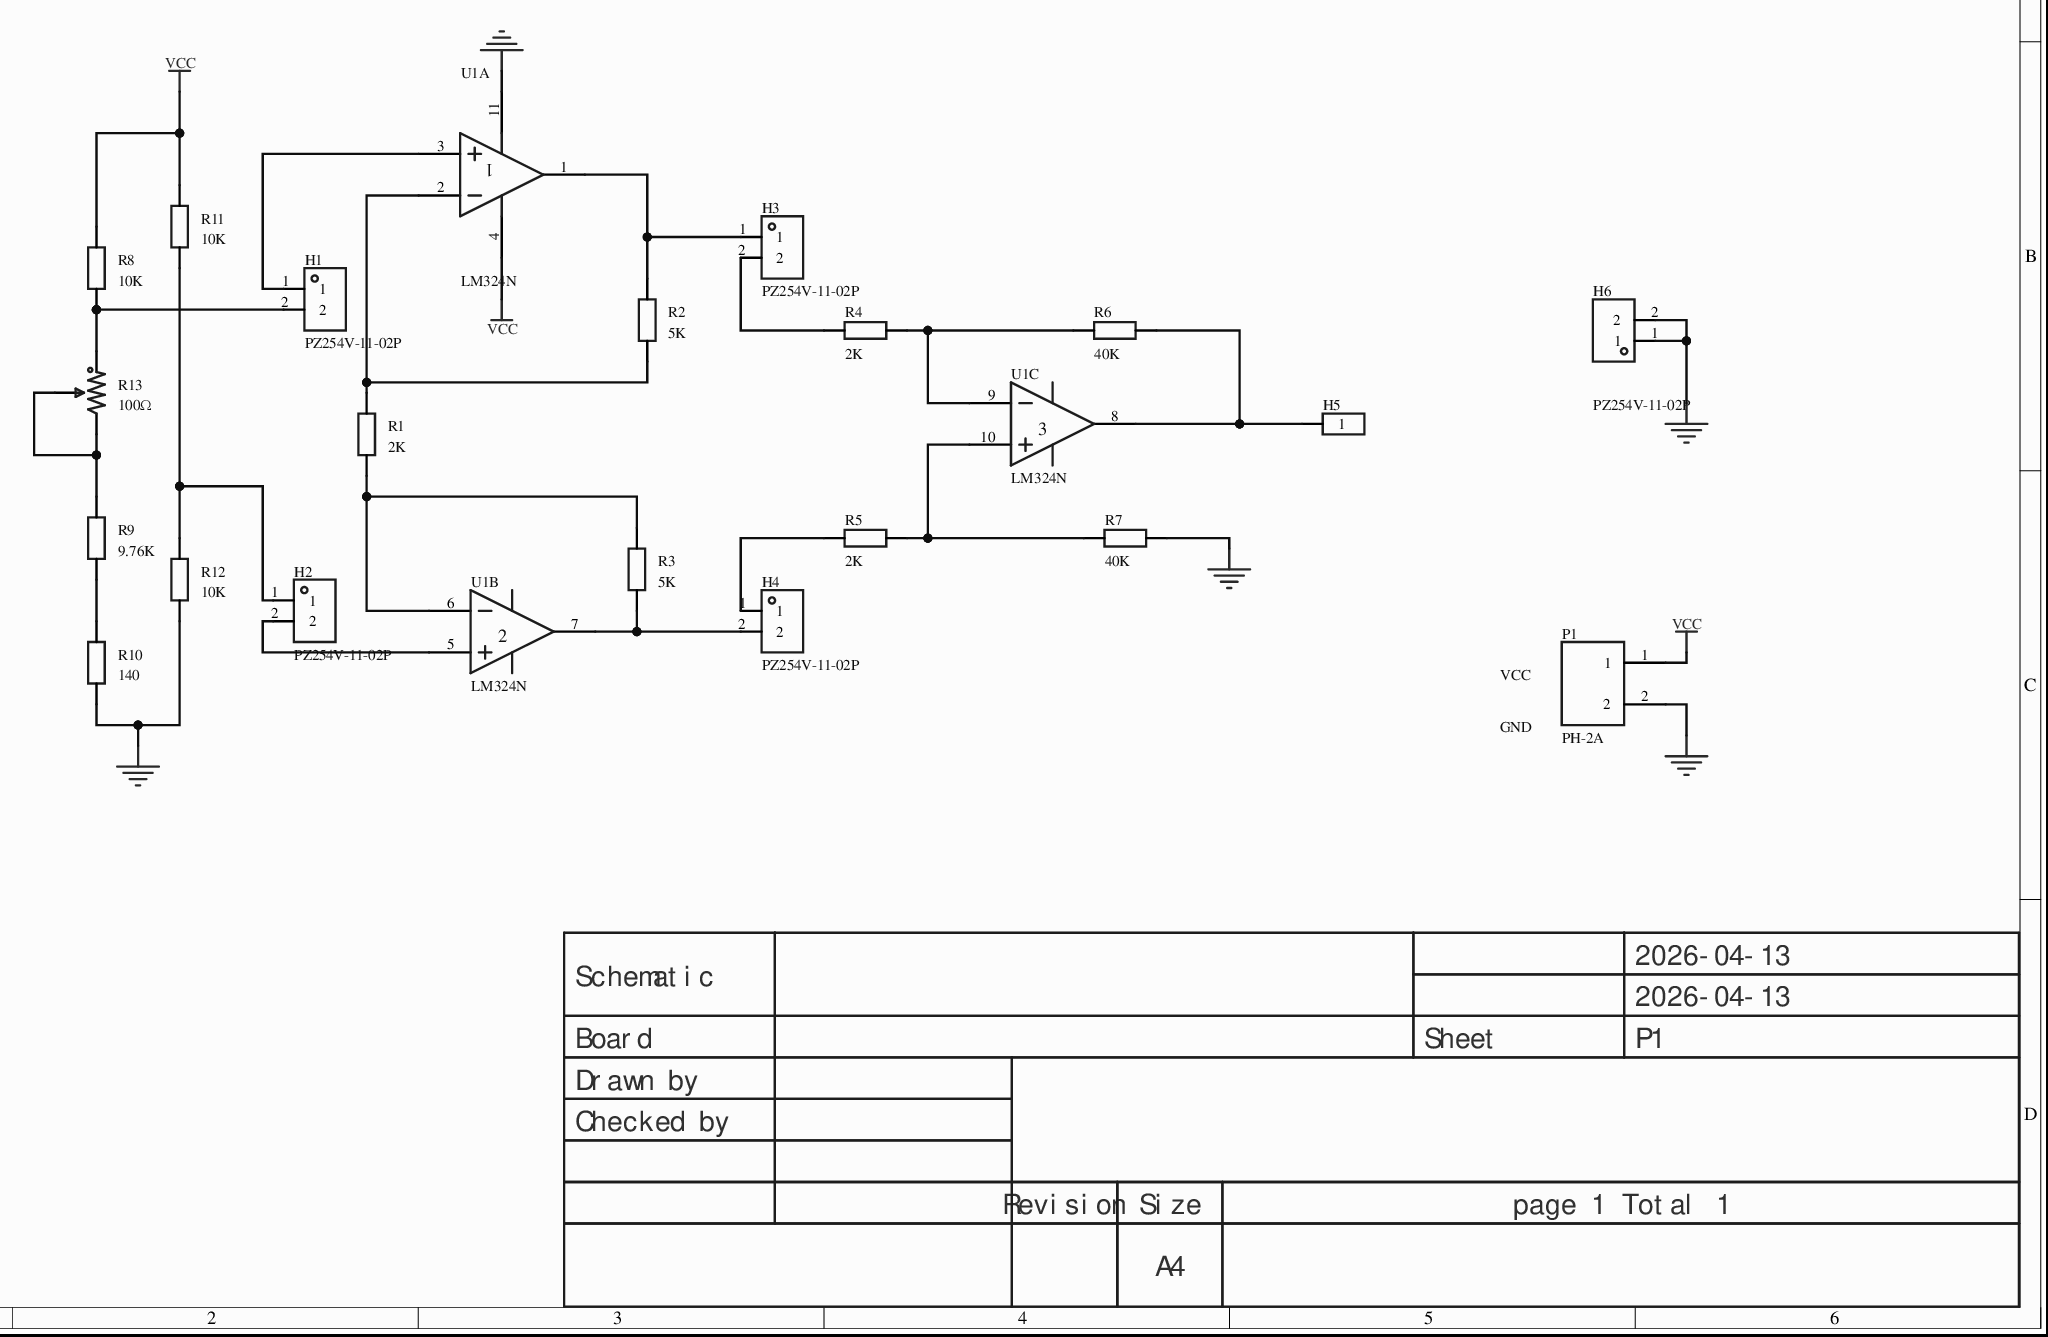
[diagram p0: MISC89092-3.schdoc]
# Altium project MISC89092-2.PrjPcb
1 sheet, 21 parts. Net scope: global (net labels, ports and power ports of the same name join across sheets).
Board file: MISC89092.pcbdoc

## Sheet MISC89092-3.schdoc
size 297 x 209 mm; Version: V1.0; @Project Name: MISC89092; @Page Count: 1; @Update Date: 2026-04-13; @Create Date: 2026-04-13; @Schematic Name: MISC89092; @Page No: 1; @Board Name: MISC89092; @Create Time: 11:14:18; @Update Time: 21:06:04; Size: A4

### Parts
H1  PZ254V-11-02P  [HDR-TH_2P-P2.54-V-M]
H2  PZ254V-11-02P  [HDR-TH_2P-P2.54-V-M]
H3  PZ254V-11-02P  [HDR-TH_2P-P2.54-V-M]
H4  PZ254V-11-02P  [HDR-TH_2P-P2.54-V-M]
H5  (no value)  [HDR-TH_1P-V-M_XKB_X4611WV-01I-C28D40]
H6  PZ254V-11-02P  [HDR-TH_2P-P2.54-V-M]
P1  PH-2A  [CONN-TH_2P-P2.00_PH-2A_C2319]
R1  2K  [R0805_1]
R2  5K  [R0805_1]
R3  5K  [R0805_1]
R4  2K  [R0805_1]
R5  2K  [R0805_1]
R6  40K  [R0805_1]
R7  40K  [R0805_1]
R8  10K  [R0805_1]
R9  9.76K  [R0805_1]
R10  140  [R0805_1]
R11  10K  [R0805_1]
R12  10K  [R0805_1]
R13  100Ω  [RES-ADJ-TH_3296W]
U1  LM324N  [DIP-14_L19.4-W6.4-P2.54-LS7.6-BL]  (parts A,B,C of 4)

### Nets
GND: H6.1 H6.2 P1.2 R7.1 R10.1 R12.1 U1.11(GND)
VCC: P1.1 R8.2 R11.2 U1.4(VCC)
NetH1_1: H1.1 U1.3(IN1+)
NetH1_2: H1.2 R8.1 R13.1
NetH2_1: H2.1 R11.1 R12.2
NetH2_2: H2.2 U1.5(IN2+)
NetH3_1: H3.1 R2.2 U1.1(OUT1)
NetH3_2: H3.2 R4.2
NetH4_1: H4.1 R5.2
NetH4_2: H4.2 R3.1 U1.7(OUT2)
NetH5_1: H5.1 R6.1 U1.8(OUT3)
NetR1_1: R1.1 R3.2 U1.6(IN2-)
NetR1_2: R1.2 R2.1 U1.2(IN1-)
NetR4_1: R4.1 R6.2 U1.9(IN3-)
NetR5_1: R5.1 R7.2 U1.10(IN3+)
NetR9_1: R9.1 R10.2
NetR9_2: R9.2 R13.2 R13.3

### Notes on the sheet
- VCC
- GND
- 2026-04-13
- Schematic
- Board
- Sheet
- P1
- Drawn by
- Checked by
- Revision
- Size
- A4
- page 1 Total 1

### Library data of the parts
H1-H4 H6 = PZ254V-11-02P: Pin structure:1x2P;Pitch:2.54mm;Row spacing:-;Round/square pins:Square;Mounting:Through-hole;Rows:Single row;Total pins:2P;Rated current:3A;Rated voltage:250V;Mating pin length:6mm;Body height:2.5mm;Tail length:3mm;Contact material:Brass;Contact plating:-;Operating temperature:-40℃~+105℃;Color:Black;; Manufacturer: XFCN(兴飞); AddInBom: yes; ModelId: e35305ec3aa84b66b849f914b715e73f; ModelName: HDR2.54-M-LI-1X2P; ModelTransform: 200,100,0,0,0,0,0,0,-118.11; Pin Structure: 1x2P; Pitch: 2.54mm; Current Rating: 3A; Voltage Rating (Max): 250V; Symbol: PZ254V-11-02P; Device: PZ254V-11-02P; LCSC Part Name: 1x2P 间距:2.54mm 方针 直插; SupplierPart: C492401; ManufacturerPart: PZ254V-11-02P; Supplier Footprint: 插件,P=2.54mm; JLCPCB Part Class: Extended library; Datasheet: https://item.szlcsc.com/datasheet/PZ254V-11-02P/502957.html; Supplier: LCSC; ConvertToPcb: yes; FootprintName: HDR-TH_2P-P2.54-V-M; Row Spacing: -; Circluar Pins/Square Pins: Square pins; Mounting Type: Through-hole; Number of Rows: Single row; Number of Pins: 2P; Length of Mating Pin: 6mm; Insulation Height: 2.5mm; Length of End Connection Pin: 3mm; Contact Material: Brass; Contact Plating: -; Operating Temperature: -40℃~+105℃; Color: Black
H5 = HDR-M_2.54_1x1P: Symbol: HDR_1x1; ConvertToPcb: yes; ModelId: 95857080d3cc4057a19a22ccce05e171; ModelTransform: 78.74,79.1337,0,0,0,0,0,0,-110.236; Device: HDR-M_2.54_1x1P; AddInBom: yes; SupplierPart: C81276; Supplier Footprint: 插件; FootprintName: HDR-TH_1P-V-M_XKB_X4611WV-01I-C28D40; JLCPCB Part Class: Extended Part; ModelName: HDR-TH_1P-V-M_XKB_X4611WV-01I-C28D40
P1 = PH-2A: Reference series:PH;Pitch:2mm;Pin structure:1x2P;Rows:1;Pins per row:2;Row spacing:-;Mounting:-;Contact material:-;; Manufacturer: BOOMELE(博穆精密); Symbol: PH-2A_C2319; AddInBom: yes; ModelId: 6e21c55398ff464d8308d4519bacd6cb; ModelName: PH2.0-LI-2P; ModelTransform: 232.283,185.039,0,0,0,0,0,-25.591,-118.11; Reference Series: PH; Pitch: 2mm; Pins Structure: 1x2P; Number of PINs Per Row: 2; Device: PH-2A; LCSC Part Name: PH-2A 2P 脚距2.0mm 直插 直插; SupplierPart: C2319; ManufacturerPart: PH-2A; Supplier Footprint: 插件,P=2mm; JLCPCB Part Class: Extended Part; Datasheet: https://atta.szlcsc.com/upload/public/pdf/source/20151208/1457707613620.pdf; Supplier: LCSC; ConvertToPcb: yes; FootprintName: CONN-TH_2P-P2.00_PH-2A_C2319; Number of Rows: 1; Row Spacing: -; Mounting Style: -; Contact Material: -
R1-R12 = Res_0603: ConvertToPcb: yes; SymbolName: Resistor; ModelId: fc143cca1e79419f9cd78b61e9279f08; ModelName: R0603; ModelTransform: 31.8897,63.7794,0,90,0,0,0,0,0; Supplier Footprint: 0805; Device: Res_0603; AddInBom: yes; FootprintName: R0805_1
  R1 R4 R5: Value: 2K
  R2 R3: Value: 5K
  R6 R7: Value: 40K
  R8 R11 R12: Value: 10K
  R9: Value: 9.76K
  R10: Value: 140
R13 = 3296W-1-101_C48997939: Resistance:100Ω;Tolerance:±10%;Power:500mW;Temperature coefficient:±250ppm/℃;; Manufacturer: JIERR(捷而瑞); AddInBom: yes; ModelId: 3664f7b541aa4725a8b6d3b7a961f078; ModelTransform: 374.015,188.976,0,90,0,0,2.362,0.005,-137.795; Tolerance: ±10%; Power(Watts): 500mW; Number of Turns: 28; Symbol: 3296W-1-101_C48997939; Device: 3296W-1-101_C48997939; LCSC Part Name: 3296W-1-101; SupplierPart: C48997939; ManufacturerPart: 3296W-1-101; Supplier Footprint: 插件-3P,9.5x4.9mm; JLCPCB Part Class: Extended library; Datasheet: https://item.szlcsc.com/datasheet/3296W-1-101/51342075.html; Supplier: LCSC; ConvertToPcb: yes; FootprintName: RES-ADJ-TH_3296W; ModelName: RES-ADJ-TH_3296W; Value: 100Ω; Temperature Coefficient: ±250ppm/℃
U1 = LM324N_C725320: Amplifier count:Quad;Rail-to-rail:-;Gain bandwidth product (GBP):-;Input offset voltage (Vos):9mV;Slew rate (SR):-;Input bias current (Ib):250nA;; Manufacturer: HGSEMI(华冠); Relevance: []; AddInBom: yes; ModelId: 4bcd59468cdc49288dfe5d29f2358061; ModelName: DIP-14_L19.4-W6.4-H5.3-P2.54-LS7.6-BL; ModelTransform: 775.19522,311.8104,0,0,0,0,0,-0.02,-118.11; Number of Channels: Quad; Maximum Power Supply Range (Vdd-Vss): 30V; Vos - Input Offset Voltage: 9mV; Input Offset Voltage Drift(Vos TC): 7uV/℃; Ib - Input Bias Current: 250nA; Input Offset Current(Ios): 50nA; Common Mode Rejection Ratio(CMRR): 80dB; Quiescent Current: 600uA; Output Current: 35mA; Single supply: 1.5V~30V; Dual Supply: -16V~-1.5V; 1.5V~16V; Symbol: LM324N_C725320; Device: LM324N_C725320; LCSC Part Name: 四路运算放大器; SupplierPart: C725320; ManufacturerPart: LM324N; Supplier Footprint: DIP-14; JLCPCB Part Class: Extended library; Datasheet: https://item.szlcsc.com/datasheet/LM324N/771554.html; Supplier: LCSC; ConvertToPcb: yes; FootprintName: DIP-14_L19.4-W6.4-P2.54-LS7.6-BL; Rail to Rail: -; Gain Bandwidth Product: -; Slew Rate: -; Noise density(eN): -; Input offset current drift(Ios TC): -; Operating Temperature: -40℃~+85℃